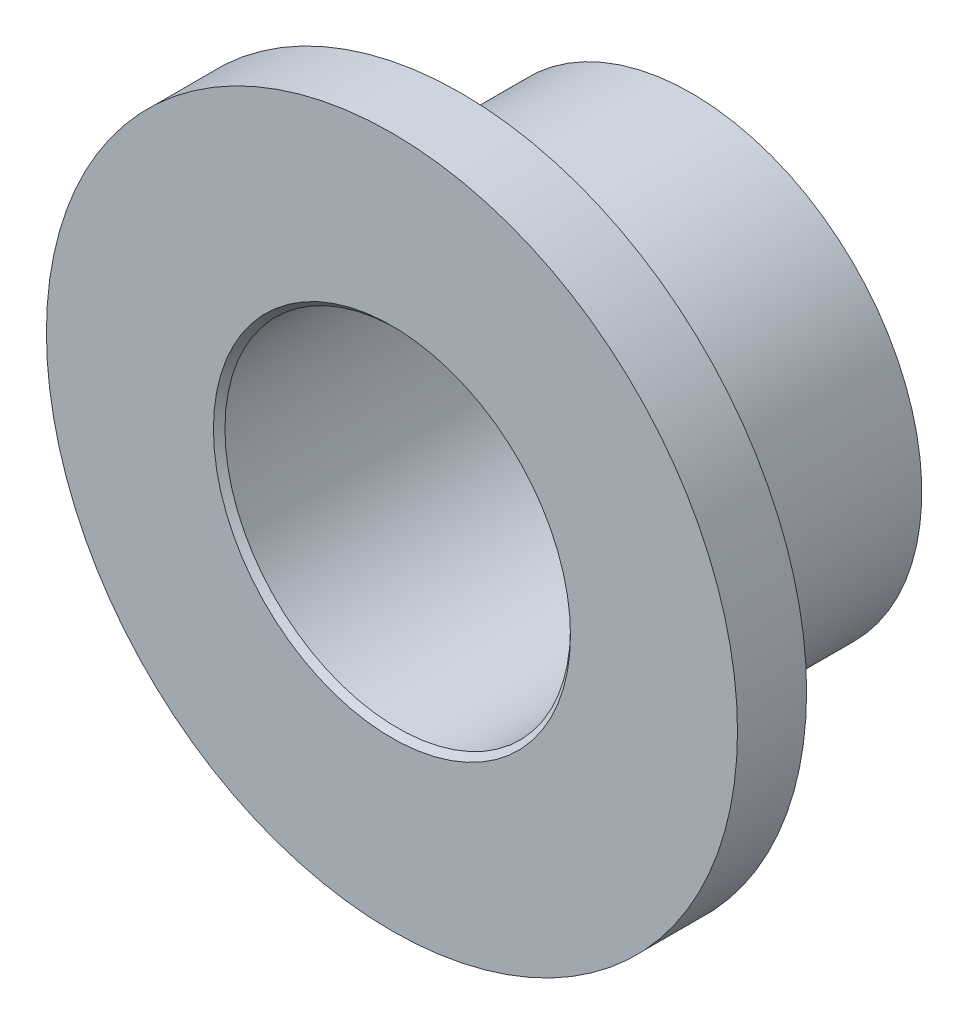
from build123d import *

# Parameters (mm, degrees)
SKETCH1_R           = 20
SKETCH1_R_2         = 15
BOSS_EXTRUDE1_DEPTH = 26
BOSS_EXTRUDE2_START = -6
SKETCH2_R           = 30
SKETCH2_R_2         = 15
BOSS_EXTRUDE2_DEPTH = 6
FILLET1_R           = 3
CHAMFER2_SIZE       = 0.5


with BuildPart() as part:
    # Sketch1 → Boss-Extrude1 (new body)
    with BuildSketch(Plane.XY):
        with Locations(Location((0, 0, 0), (0, 0, 180))):
            Circle(SKETCH1_R)
        with Locations(Location((0, 0, 0), (0, 0, 180))):
            Circle(SKETCH1_R_2, mode=Mode.SUBTRACT)
    extrude(amount=BOSS_EXTRUDE1_DEPTH)

    # Sketch2 → Boss-Extrude2 (add)
    with BuildSketch(Plane.XY.offset(26).offset(BOSS_EXTRUDE2_START)):
        Circle(SKETCH2_R)
        with Locations(Location((0, 0, 0), (0, 0, 180))):
            Circle(SKETCH2_R_2, mode=Mode.SUBTRACT)
    extrude(amount=BOSS_EXTRUDE2_DEPTH)

    # Fillet1
    fillet1_edges = [part.edges().sort_by_distance(p)[0] for p in [
        (20, 0, 20),
    ]]
    fillet(fillet1_edges, radius=FILLET1_R)

    # Chamfer2
    chamfer2_edges = [part.edges().sort_by_distance(p)[0] for p in [
        (15, 0, 0),
        (15, 0, 26),
    ]]
    chamfer(chamfer2_edges, length=CHAMFER2_SIZE)


solid = part.part
